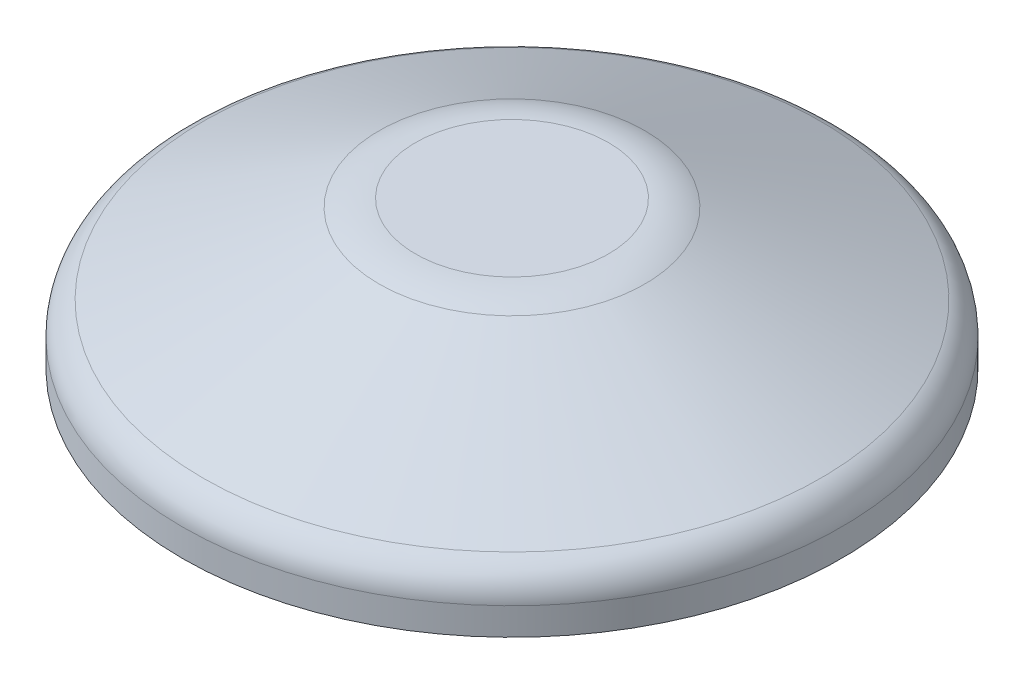
from build123d import *

# Parameters (mm, degrees)
FILLET1_R = 40
FILLET2_R = 38
FILLET3_R = 16
FILLET4_R = 4


with BuildPart() as part:
    # Sketch1 → Revolve1 (revolve)
    with BuildSketch(Plane.XY, mode=Mode.PRIVATE) as revolve1_sk:
        Polygon((-150, 1.447982474), (-150, 24.174941718), (-52.599310337, 68.447982474), (0, 68.447982474), (0, 56.447982474), (-50, 56.447982474), (-132, 19.175255201), (-132, 1.447982474), (-132, -4.552017526), (-138, -4.552017526), (-138, 1.447982474), align=None)
    revolve(revolve1_sk.sketch.rotate(Axis((0, 0, 0), (0, 1, 0)), 270), axis=Axis((0, 0, 0), (0, 1, 0)))

    # Fillet1
    fillet1_edges = [part.edges().sort_by_distance(p)[0] for p in [
        (0, 68.447982474, 52.599310337),
    ]]
    fillet(fillet1_edges, radius=FILLET1_R)

    # Fillet2
    fillet2_edges = [part.edges().sort_by_distance(p)[0] for p in [
        (0, 56.447982474, 50),
    ]]
    fillet(fillet2_edges, radius=FILLET2_R)

    # Fillet3
    fillet3_edges = [part.edges().sort_by_distance(p)[0] for p in [
        (0, 24.174941718, 150),
    ]]
    fillet(fillet3_edges, radius=FILLET3_R)

    # Fillet4
    fillet4_edges = [part.edges().sort_by_distance(p)[0] for p in [
        (0, 19.175255201, 132),
    ]]
    fillet(fillet4_edges, radius=FILLET4_R)


solid = part.part
